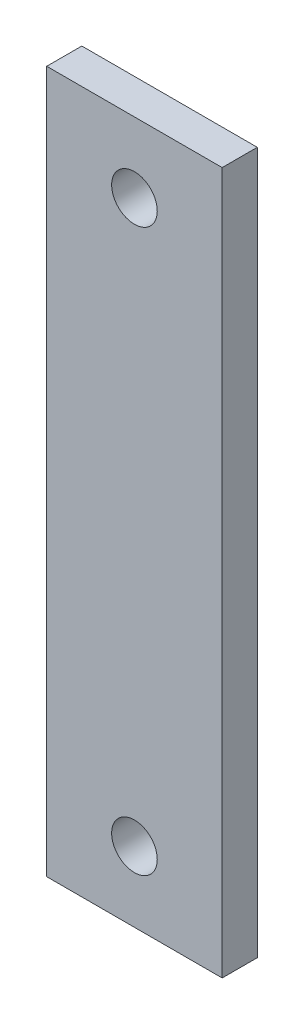
from build123d import *

# Parameters (mm, degrees)
SKETCH_1_W      = 50
SKETCH_1_H      = 200
SKETCH_1_R      = 6.5
EXTRUDE_1_DEPTH = 10


with BuildPart() as part:
    # 草图1 → 凸台-拉伸1 (new body)
    with BuildSketch(Plane.XY):
        Rectangle(SKETCH_1_W, SKETCH_1_H)
        with Locations((0, 80)):
            Circle(SKETCH_1_R, mode=Mode.SUBTRACT)
        with Locations((0, -80)):
            Circle(SKETCH_1_R, mode=Mode.SUBTRACT)
    extrude(amount=EXTRUDE_1_DEPTH)


solid = part.part
